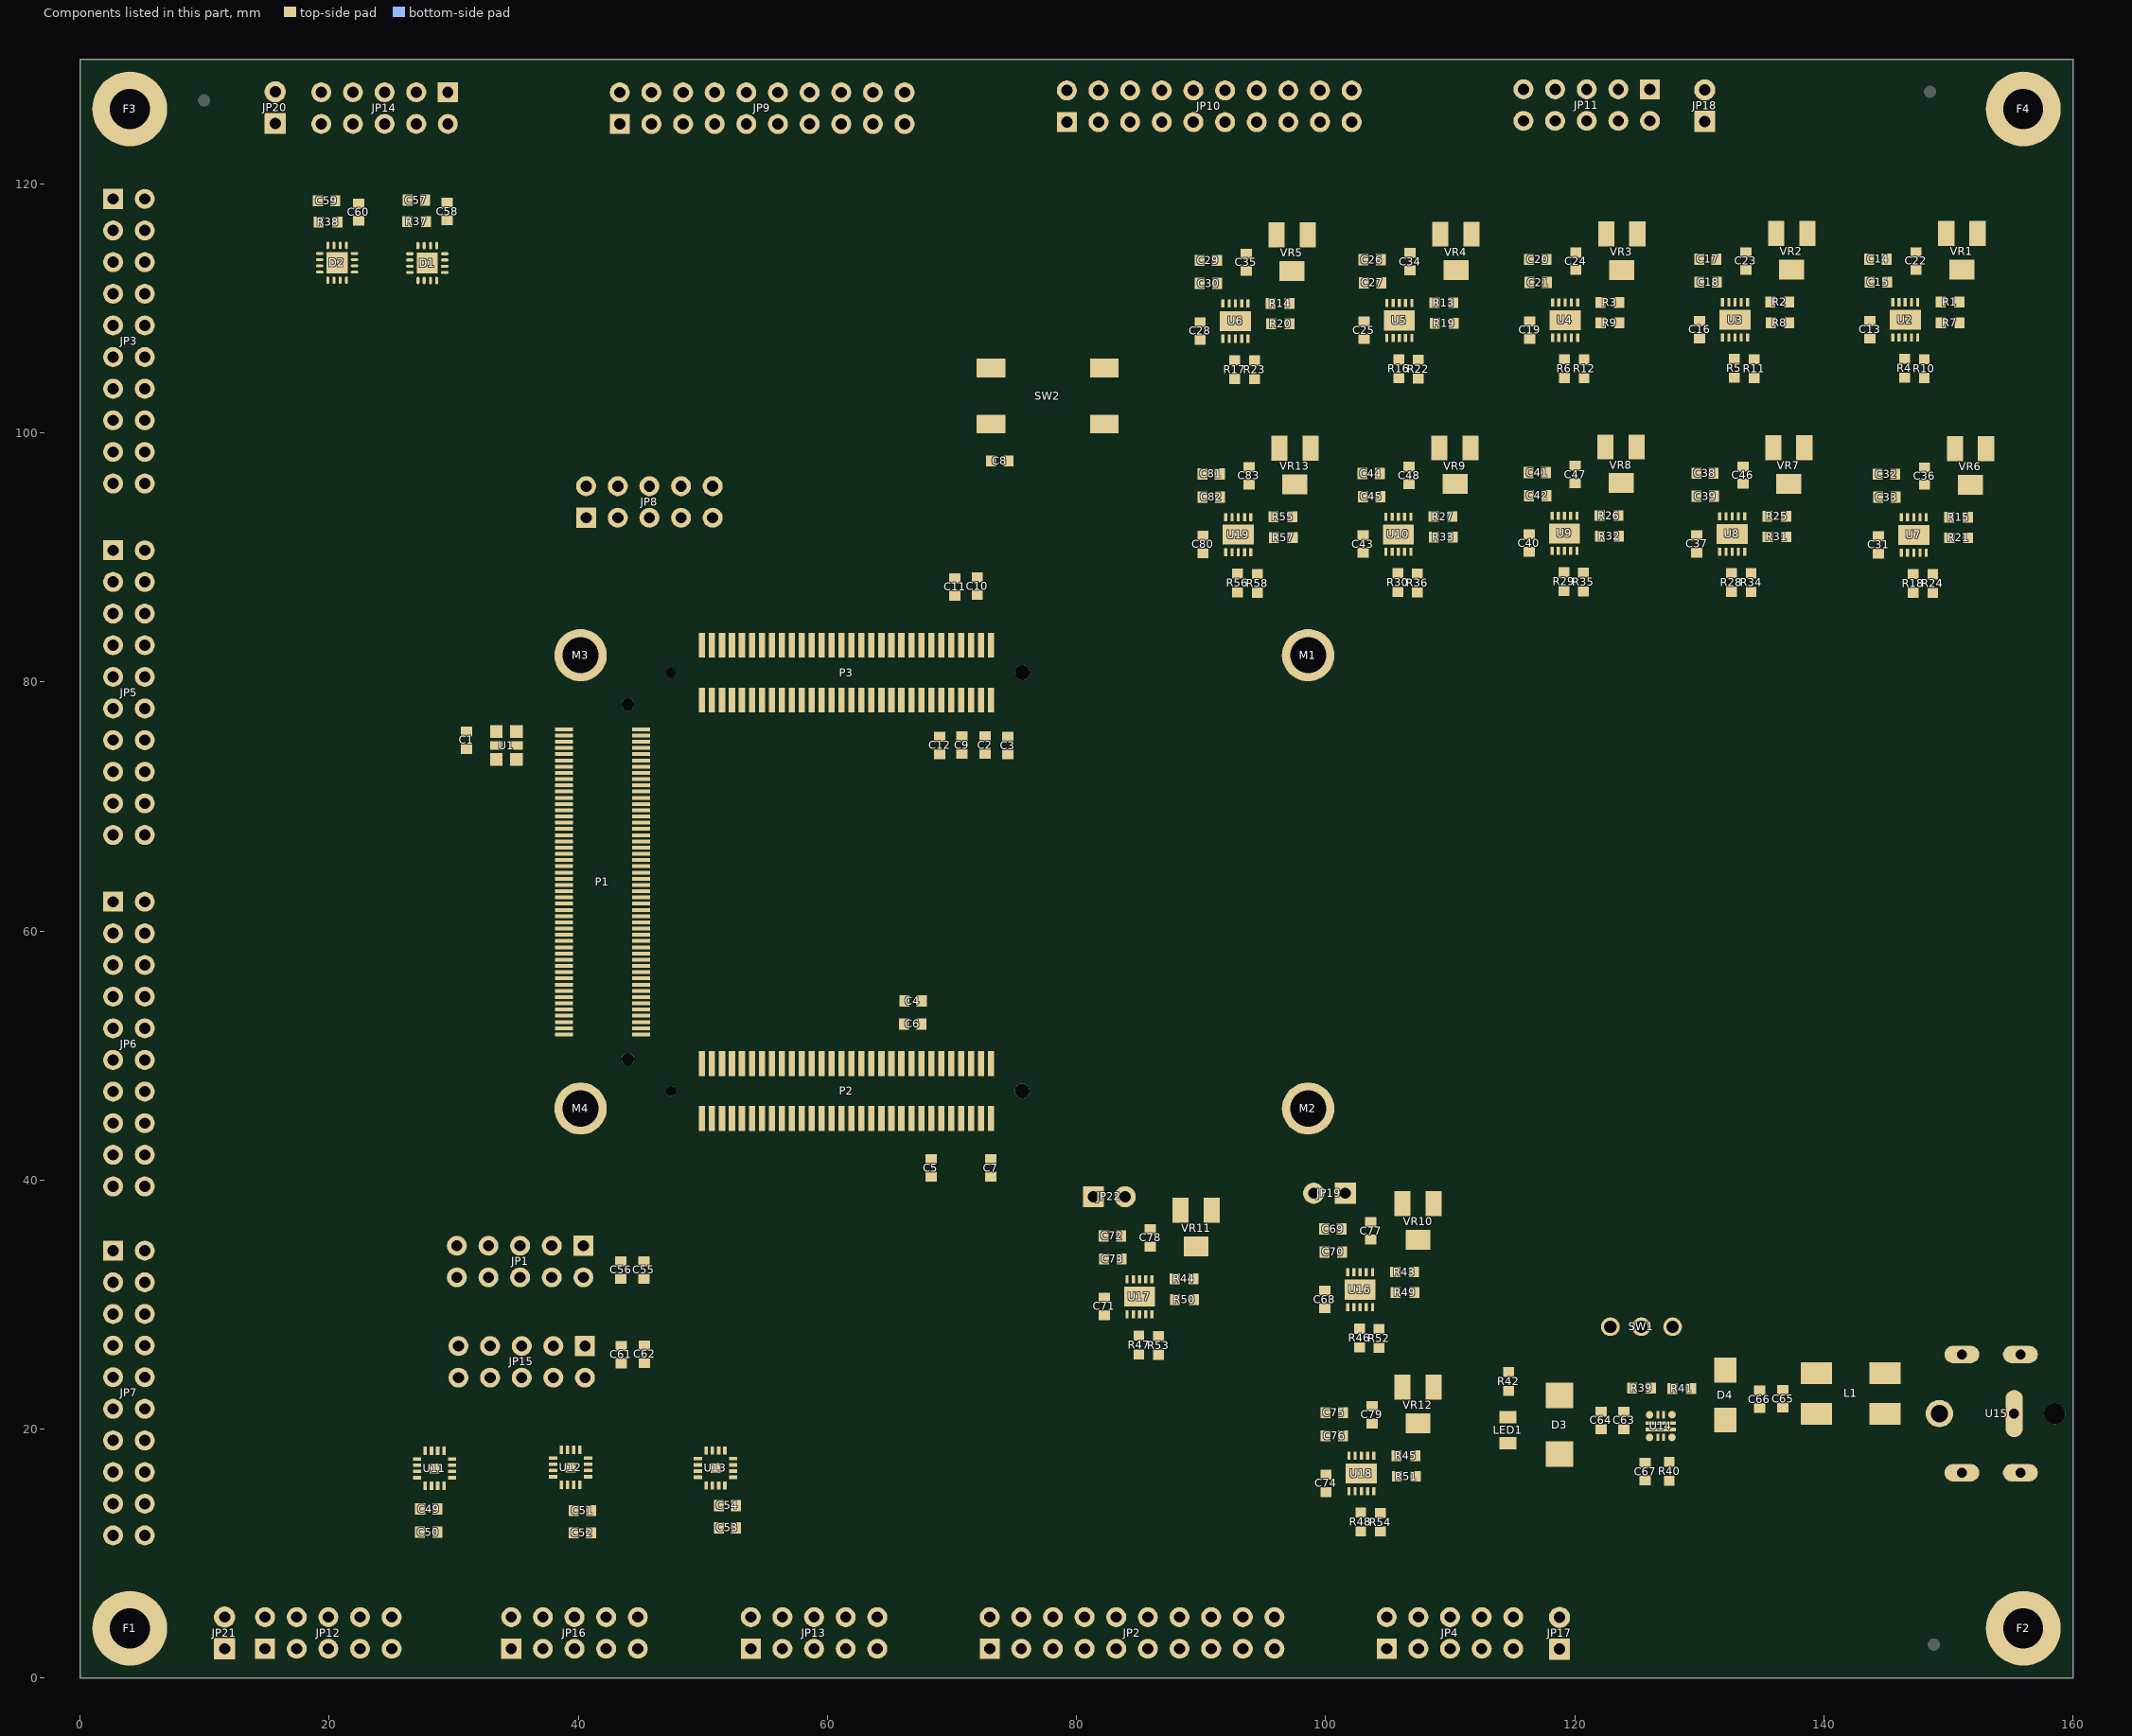
[diagram p0: the components of this part, seen from the top]
# Altium PCB MISC82195.PcbDoc (part 8 of 8)
Units mm, origin at the board's own origin, x right, y up, seen from the top; angles counter-clockwise.
Board outline 160 x 130 mm, 4 copper layers (Top Layer, GND, POWER, Bottom Layer); 214 components, 251 nets, 1068 pads, 1218 vias.

## Silkscreen, mask and mechanical layers (free items; w line width, h text height)
Top Overlay:
  lines w0.3: 37.387,42.939 101.387,42.939 101.387,84.938 37.387,84.938 37.387,42.939
  text "GND" at 18.085,122.377 h1.02
  text "GND" at 21.133,122.352 h1.02
  text "LDO10" at 25.654,122.352 h1.02
  text "1V8" at 29.159,122.326 h1.02
  text "GND" at 15.9,121.463 h1.02 r90
  text "GND" at 24.841,121.437 h1.02 r90
  text "GND" at 100,121.412 h1.02 r90
  text "GND" at 97.307,121.336 h1.02 r90
  text "GND" at 102.21,121.336 h1.02 r90
  text "GND" at 130.886,121.31 h1.02 r90
  text "LDO2" at 123.876,121.26 h1.02 r90
  text "LDO1" at 126.492,121.26 h1.02 r90
  text "LDO3" at 121.336,121.234 h1.02 r90
  text "LDO5" at 116.154,121.183 h1.02 r90
  text "LDO4" at 118.72,121.107 h1.02 r90
  text "1OUT0" at 25.552,120.853 h1.02
  text "1OUT1" at 29.032,120.777 h1.02
  text "2OUT1" at 20.625,120.625 h1.02
  text "2OUT0" at 17.272,120.574 h1.02
  text "PW120" at 89.637,120.523 h1.02 r90
  text "PW119" at 92.075,120.498 h1.02 r90
  text "PW118" at 94.64,120.498 h1.02 r90
  text "PW122" at 84.506,120.447 h1.02 r90
  text "PW121" at 87.097,120.447 h1.02 r90
  text "PW123" at 82.017,120.371 h1.02 r90
  text "PW124" at 79.4,120.218 h1.02 r90
  text "PW126" at 64.211,119.964 h1.02 r90
  text "PW132" at 48.92,119.913 h1.02 r90
  text "PW130" at 54.051,119.913 h1.02 r90
  text "PW125" at 66.396,119.913 h1.02 r90
  text "PW129" at 56.49,119.888 h1.02 r90
  text "PW128" at 59.055,119.888 h1.02 r90
  text "PW127" at 61.595,119.888 h1.02 r90
  text "PW131" at 51.384,119.837 h1.02 r90
  text "PW134" at 43.866,119.812 h1.02 r90
  text "PW133" at 46.431,119.761 h1.02 r90
  text "GND" at 15.926,119.329 h1.02 r90
  text "VDD" at 24.841,119.329 h1.02 r90
  text "GND" at 130.861,118.897 h1.02 r90
  text "LDO7" at 123.952,118.593 h1.02 r90
  text "LDO6" at 126.594,118.567 h1.02 r90
  text "PW29" at 10.592,118.516 h1.02
  text "PW28" at 7.137,118.466 h1.02
  text "LDO8" at 121.387,118.389 h1.02 r90
  text "LDO9" at 118.847,118.288 h1.02 r90
  text "GND" at 102.26,118.034 h1.02 r90
  text "LDO10" at 116.281,117.983 h1.02 r90
  text "GND" at 97.434,117.881 h1.02 r90
  text "GND" at 100.076,117.856 h1.02 r90
  text "GND" at 94.615,117.78 h1.02 r90
  text "PW113" at 82.067,116.891 h1.02 r90
  text "PW117" at 92.126,116.891 h1.02 r90
  text "PW116" at 89.713,116.865 h1.02 r90
  text "PW114" at 84.557,116.84 h1.02 r90
  text "PW115" at 87.173,116.815 h1.02 r90
  text "PW112" at 79.502,116.764 h1.02 r90
  text "PW102" at 43.84,116.307 h1.02 r90
  text "PW111" at 66.446,116.307 h1.02 r90
  text "PW103" at 46.482,116.281 h1.02 r90
  text "PW107" at 56.54,116.281 h1.02 r90
  text "PW109" at 61.595,116.281 h1.02 r90
  text "PW110" at 64.186,116.281 h1.02 r90
  text "PW106" at 54.026,116.256 h1.02 r90
  text "PW104" at 48.971,116.23 h1.02 r90
  text "PW108" at 59.131,116.23 h1.02 r90
  text "PW105" at 51.359,116.205 h1.02 r90
  text "PW31" at 10.465,116.078 h1.02
  text "PW30" at 7.01,115.951 h1.02
  text "PW33" at 10.617,113.436 h1.02
  text "PW32" at 7.137,113.386 h1.02
  text "PW35" at 10.693,110.947 h1.02
  text "PW34" at 7.087,110.896 h1.02
  text "GND" at 7.163,108.229 h1.02
  text "GND" at 10.77,108.204 h1.02
  text "PW36" at 7.112,105.842 h1.02
  text "PW37" at 10.77,105.816 h1.02
  text "PW95" at 10.744,103.378 h1.02
  text "PW94" at 7.137,103.327 h1.02
  text "PW97" at 10.744,100.813 h1.02
  text "PW96" at 7.087,100.736 h1.02
  text "PW99" at 10.82,98.374 h1.02
  text "PW98" at 7.137,98.273 h1.02
  text "PW100" at 7.137,95.733 h1.02
  text "PW101" at 10.82,95.656 h1.02
  text "PW93" at 10.846,90.094 h1.02
  text "PW38" at 7.391,89.992 h1.02
  text "PW92" at 10.998,87.478 h1.02
  text "PW39" at 7.518,87.427 h1.02
  text "PW91" at 11.074,84.988 h1.02
  text "PW40" at 7.468,84.938 h1.02
  text "PW90" at 11.049,82.601 h1.02
  text "PW41" at 7.442,82.55 h1.02
  text "PW42" at 7.493,79.883 h1.02
  text "PW89" at 11.151,79.858 h1.02
  text "PW88" at 11.125,77.419 h1.02
  text "PW43" at 7.518,77.368 h1.02
  text "PW87" at 11.125,74.854 h1.02
  text "PW44" at 7.468,74.778 h1.02
  text "PW86" at 11.201,72.415 h1.02
  text "PW45" at 7.518,72.314 h1.02
  text "PW46" at 7.518,69.774 h1.02
  text "PW85" at 11.201,69.698 h1.02
  text "PW84" at 11.151,67.513 h1.02
  text "PW47" at 7.544,67.462 h1.02
  text "PW83" at 11.328,62.078 h1.02
  text "PW48" at 7.874,61.976 h1.02
  text "PW82" at 11.481,59.461 h1.02
  text "PW49" at 8.001,59.411 h1.02
  text "PW81" at 11.557,56.972 h1.02
  text "PW50" at 7.95,56.921 h1.02
  text "PW80" at 11.532,54.585 h1.02
  text "PW51" at 7.925,54.534 h1.02
  text "PW52" at 7.976,51.867 h1.02
  text "PW79" at 11.633,51.841 h1.02
  text "PW78" at 11.608,49.403 h1.02
  text "PW53" at 8.001,49.352 h1.02
  text "PW77" at 11.608,46.838 h1.02
  text "PW54" at 7.95,46.761 h1.02
  text "PW76" at 11.684,44.399 h1.02
  text "PW55" at 8.001,44.298 h1.02
  text "PW56" at 8.001,41.758 h1.02
  text "PW75" at 11.684,41.681 h1.02
  text "PW74" at 11.633,39.472 h1.02
  text "PW57" at 8.026,39.446 h1.02
  text "PW73" at 11.252,33.909 h1.02
  text "PW58" at 7.798,33.807 h1.02
  text "PW72" at 11.405,31.293 h1.02
  text "PW59" at 7.925,31.242 h1.02
  text "PW71" at 11.481,28.804 h1.02
  text "PW60" at 7.874,28.753 h1.02
  text "PW70" at 11.455,26.416 h1.02
  text "PW61" at 7.849,26.365 h1.02
  text "PW62" at 7.899,23.698 h1.02
  text "PW69" at 11.557,23.673 h1.02
  text "PW68" at 11.532,21.234 h1.02
  text "PW63" at 7.925,21.184 h1.02
  text "PW67" at 11.532,18.669 h1.02
  text "PW64" at 7.874,18.593 h1.02
  text "PW66" at 11.608,16.231 h1.02
  text "GND" at 7.925,16.129 h1.02
  text "GND" at 7.925,13.589 h1.02
  text "PW65" at 11.608,13.513 h1.02
  text "GND" at 11.557,11.328 h1.02
  text "GND" at 7.95,11.278 h1.02
  text "PW20" at 91.186,10.592 h1.02 r90
  text "PW23" at 83.744,10.541 h1.02 r90
  text "PW18" at 96.114,10.541 h1.02 r90
  text "PW22" at 86.182,10.516 h1.02 r90
  text "PW21" at 88.748,10.516 h1.02 r90
  text "PW25" at 78.613,10.465 h1.02 r90
  text "PW24" at 81.001,10.439 h1.02 r90
  text "PW19" at 93.751,10.439 h1.02 r90
  text "PW26" at 76.124,10.389 h1.02 r90
  text "PW27" at 73.508,10.236 h1.02 r90
  text "3OUT2" at 56.566,9.881 h1.02 r90
  text "3OUT6" at 61.747,9.804 h1.02 r90
  text "GND" at 64.287,9.804 h1.02 r90
  text "1OUT6" at 22.809,9.728 h1.02 r90
  text "1OUT4" at 20.066,9.703 h1.02 r90
  text "2OUT2" at 37.465,9.652 h1.02 r90
  text "3OUT0" at 54.432,9.627 h1.02 r90
  text "3OUT4" at 59.004,9.627 h1.02 r90
  text "1OUT2" at 17.704,9.601 h1.02 r90
  text "1OUT0" at 15.088,9.576 h1.02 r90
  text "2OUT0" at 34.722,9.576 h1.02 r90
  text "PW17" at 105.918,9.373 h1.02 r90
  text "PW15" at 110.033,9.347 h1.02 r90
  text "PW16" at 107.671,9.296 h1.02 r90
  text "PW14" at 112.979,9.271 h1.02 r90
  text "GND" at 119.177,9.22 h1.02 r90
  text "GND" at 115.341,9.068 h1.02 r90
  text "GND" at 11.836,9.017 h1.02 r90
  text "GND" at 45.288,9.017 h1.02 r90
  text "GND" at 25.349,8.941 h1.02 r90
  text "2OUT6" at 41.529,8.23 h1.02
  text "2OUT4" at 38.329,8.128 h1.02
  text "PW10" at 96.139,6.934 h1.02 r90
  text "PW2" at 76.175,6.909 h1.02 r90
  text "PW6" at 86.233,6.909 h1.02 r90
  text "PW8" at 91.288,6.909 h1.02 r90
  text "PW9" at 93.828,6.909 h1.02 r90
  text "PW5" at 83.718,6.883 h1.02 r90
  text "PW3" at 78.664,6.858 h1.02 r90
  text "PW7" at 88.824,6.858 h1.02 r90
  text "2OUT5" at 38.227,6.833 h1.02
  text "PW4" at 81.051,6.833 h1.02 r90
  text "GND" at 119.151,6.807 h1.02 r90
  text "2OUT7" at 41.504,6.782 h1.02
  text "PW1" at 73.609,6.782 h1.02 r90
  text "GND" at 115.316,6.655 h1.02 r90
  text "GND" at 45.263,6.604 h1.02 r90
  text "GND" at 11.887,6.553 h1.02 r90
  text "GND" at 64.287,6.553 h1.02 r90
  text "PW11" at 105.181,6.553 h1.02 r90
  text "GND" at 25.4,6.477 h1.02 r90
  text "GND" at 112.928,6.477 h1.02 r90
  text "1OUT5" at 20.142,6.452 h1.02 r90
  text "1OUT1" at 15.113,6.401 h1.02 r90
  text "1OUT3" at 17.729,6.401 h1.02 r90
  text "1OUT7" at 22.86,6.401 h1.02 r90
  text "2OUT1" at 34.773,6.401 h1.02 r90
  text "3OUT1" at 54.458,6.375 h1.02 r90
  text "PW12" at 107.671,6.375 h1.02 r90
  text "PW13" at 110.211,6.375 h1.02 r90
  text "2OUT3" at 37.44,6.35 h1.02 r90
  text "3OUT3" at 56.693,6.35 h1.02 r90
  text "3OUT7" at 61.773,6.35 h1.02 r90
  text "3OUT5" at 59.004,6.325 h1.02 r90